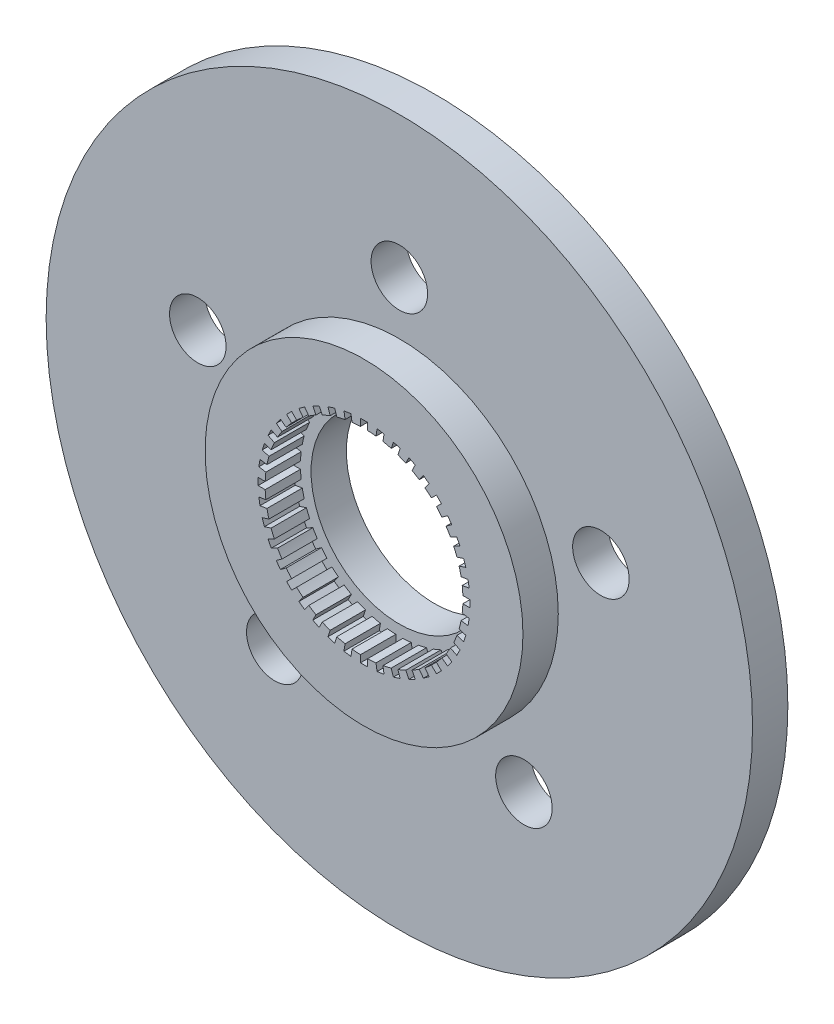
SolidWorks part; units mm, degrees
ref_plane "Front" through (0, 0, 0) normal (0, 0, 1) x (1, 0, 0)
ref_plane "Top" through (0, 0, 0) normal (0, 1, 0) x (1, 0, 0)
ref_plane "Right" through (0, 0, 0) normal (1, 0, 0) x (0, 0, -1)
sketch "草图1" plane through (0, 0, 0) normal (0, 0, 1) x (1, 0, 0)
  circle A0 centre (0, 0) radius 100
  circle A1 centre (0, 0) radius 25
  circle A2 centre (0, 60) radius 8
  circle A3 centre (57.0634, 18.541) radius 8
  circle A4 centre (35.2671, -48.541) radius 8
  circle A5 centre (-35.2671, -48.541) radius 8
  circle A6 centre (-57.0634, 18.541) radius 8
  point P17 (0, 0)
  dimension "D1" = 60
  dimension "D2" = 200
  dimension "D3" = 50
  dimension "D4" = 5
extrude "凸台-拉伸1" add sketch "草图1" along normal blind 10
sketch "草图2" plane through (0, 0, 10) normal (0, 0, 1) x (1, 0, 0)
  line L82 (3.3897, 27.7941) -> (3.7027, 29.7706)
  line L83 (-1, 27.9821) -> (-1, 29.9833)
  line L84 (-1, 29.9833) -> (1, 29.9833)
  line L85 (1, 29.9833) -> (1, 27.9821)
  line L86 (5.6781, 29.4577) -> (5.3651, 27.4812)
  line L87 (7.6959, 26.9216) -> (8.3143, 28.8249)
  line L88 (10.2164, 28.2068) -> (9.598, 26.3036)
  line L89 (11.8126, 25.3863) -> (12.7211, 27.1693)
  line L90 (14.5032, 26.2614) -> (13.5946, 24.4783)
  line L91 (15.6385, 23.2258) -> (16.8147, 24.8448)
  line L92 (18.4328, 23.6692) -> (17.2565, 22.0502)
  line L93 (19.0793, 20.4935) -> (20.4943, 21.9085)
  line L94 (21.9085, 20.4943) -> (20.4935, 19.0793)
  line L95 (22.0502, 17.2565) -> (23.6692, 18.4328)
  line L96 (24.8448, 16.8147) -> (23.2258, 15.6385)
  line L97 (24.4783, 13.5946) -> (26.2614, 14.5032)
  line L98 (27.1693, 12.7211) -> (25.3863, 11.8126)
  line L99 (26.3036, 9.598) -> (28.2068, 10.2164)
  line L100 (28.8249, 8.3143) -> (26.9216, 7.6959)
  line L101 (27.4812, 5.3651) -> (29.4577, 5.6781)
  line L102 (29.7706, 3.7027) -> (27.7941, 3.3897)
  line L103 (27.9821, 1) -> (29.9833, 1)
  line L104 (29.9833, -1) -> (27.9821, -1)
  line L105 (27.7941, -3.3897) -> (29.7706, -3.7027)
  line L106 (29.4577, -5.6781) -> (27.4812, -5.3651)
  line L107 (26.9216, -7.6959) -> (28.8249, -8.3143)
  line L108 (28.2068, -10.2164) -> (26.3036, -9.598)
  line L109 (25.3863, -11.8126) -> (27.1693, -12.7211)
  line L110 (26.2614, -14.5032) -> (24.4783, -13.5946)
  line L111 (23.2258, -15.6385) -> (24.8448, -16.8147)
  line L112 (23.6692, -18.4328) -> (22.0502, -17.2565)
  line L113 (20.4935, -19.0793) -> (21.9085, -20.4943)
  line L114 (20.4943, -21.9085) -> (19.0793, -20.4935)
  line L115 (17.2565, -22.0502) -> (18.4328, -23.6692)
  line L116 (16.8147, -24.8448) -> (15.6385, -23.2258)
  line L117 (13.5946, -24.4783) -> (14.5032, -26.2614)
  line L118 (12.7211, -27.1693) -> (11.8126, -25.3863)
  line L119 (9.598, -26.3036) -> (10.2164, -28.2068)
  line L120 (8.3143, -28.8249) -> (7.6959, -26.9216)
  line L121 (5.3651, -27.4812) -> (5.6781, -29.4577)
  line L122 (3.7027, -29.7706) -> (3.3897, -27.7941)
  line L123 (1, -27.9821) -> (1, -29.9833)
  line L124 (-1, -29.9833) -> (-1, -27.9821)
  line L125 (-3.3897, -27.7941) -> (-3.7027, -29.7706)
  line L126 (-5.6781, -29.4577) -> (-5.3651, -27.4812)
  line L127 (-7.6959, -26.9216) -> (-8.3143, -28.8249)
  line L128 (-10.2164, -28.2068) -> (-9.598, -26.3036)
  line L129 (-11.8126, -25.3863) -> (-12.7211, -27.1693)
  line L130 (-14.5032, -26.2614) -> (-13.5946, -24.4783)
  line L131 (-15.6385, -23.2258) -> (-16.8147, -24.8448)
  line L132 (-18.4328, -23.6692) -> (-17.2565, -22.0502)
  line L133 (-19.0793, -20.4935) -> (-20.4943, -21.9085)
  line L134 (-21.9085, -20.4943) -> (-20.4935, -19.0793)
  line L135 (-22.0502, -17.2565) -> (-23.6692, -18.4328)
  line L136 (-24.8448, -16.8147) -> (-23.2258, -15.6385)
  line L137 (-24.4783, -13.5946) -> (-26.2614, -14.5032)
  line L138 (-27.1693, -12.7211) -> (-25.3863, -11.8126)
  line L139 (-26.3036, -9.598) -> (-28.2068, -10.2164)
  line L140 (-28.8249, -8.3143) -> (-26.9216, -7.6959)
  line L141 (-27.4812, -5.3651) -> (-29.4577, -5.6781)
  line L142 (-29.7706, -3.7027) -> (-27.7941, -3.3897)
  line L143 (-27.9821, -1) -> (-29.9833, -1)
  line L144 (-29.9833, 1) -> (-27.9821, 1)
  line L145 (-27.7941, 3.3897) -> (-29.7706, 3.7027)
  line L146 (-29.4577, 5.6781) -> (-27.4812, 5.3651)
  line L147 (-26.9216, 7.6959) -> (-28.8249, 8.3143)
  line L148 (-28.2068, 10.2164) -> (-26.3036, 9.598)
  line L149 (-25.3863, 11.8126) -> (-27.1693, 12.7211)
  line L150 (-26.2614, 14.5032) -> (-24.4783, 13.5946)
  line L151 (-23.2258, 15.6385) -> (-24.8448, 16.8147)
  line L152 (-23.6692, 18.4328) -> (-22.0502, 17.2565)
  line L153 (-20.4935, 19.0793) -> (-21.9085, 20.4943)
  line L154 (-20.4943, 21.9085) -> (-19.0793, 20.4935)
  line L155 (-17.2565, 22.0502) -> (-18.4328, 23.6692)
  line L156 (-16.8147, 24.8448) -> (-15.6385, 23.2258)
  line L157 (-13.5946, 24.4783) -> (-14.5032, 26.2614)
  line L158 (-12.7211, 27.1693) -> (-11.8126, 25.3863)
  line L159 (-9.598, 26.3036) -> (-10.2164, 28.2068)
  line L160 (-8.3143, 28.8249) -> (-7.6959, 26.9216)
  line L161 (-5.3651, 27.4812) -> (-5.6781, 29.4577)
  line L162 (-3.7027, 29.7706) -> (-3.3897, 27.7941)
  line L163 (3.7027, 29.7706) -> (5.6781, 29.4577)
  line L164 (8.3143, 28.8249) -> (10.2164, 28.2068)
  line L165 (12.7211, 27.1693) -> (14.5032, 26.2614)
  line L166 (16.8147, 24.8448) -> (18.4328, 23.6692)
  line L167 (20.4943, 21.9085) -> (21.9085, 20.4943)
  line L168 (23.6692, 18.4328) -> (24.8448, 16.8147)
  line L169 (26.2614, 14.5032) -> (27.1693, 12.7211)
  line L170 (28.2068, 10.2164) -> (28.8249, 8.3143)
  line L171 (29.4577, 5.6781) -> (29.7706, 3.7027)
  line L172 (29.9833, 1) -> (29.9833, -1)
  line L173 (29.7706, -3.7027) -> (29.4577, -5.6781)
  line L174 (28.8249, -8.3143) -> (28.2068, -10.2164)
  line L175 (27.1693, -12.7211) -> (26.2614, -14.5032)
  line L176 (24.8448, -16.8147) -> (23.6692, -18.4328)
  line L177 (21.9085, -20.4943) -> (20.4943, -21.9085)
  line L178 (18.4328, -23.6692) -> (16.8147, -24.8448)
  line L179 (14.5032, -26.2614) -> (12.7211, -27.1693)
  line L180 (10.2164, -28.2068) -> (8.3143, -28.8249)
  line L181 (5.6781, -29.4577) -> (3.7027, -29.7706)
  line L182 (1, -29.9833) -> (-1, -29.9833)
  line L183 (-3.7027, -29.7706) -> (-5.6781, -29.4577)
  line L184 (-8.3143, -28.8249) -> (-10.2164, -28.2068)
  line L185 (-12.7211, -27.1693) -> (-14.5032, -26.2614)
  line L186 (-16.8147, -24.8448) -> (-18.4328, -23.6692)
  line L187 (-20.4943, -21.9085) -> (-21.9085, -20.4943)
  line L188 (-23.6692, -18.4328) -> (-24.8448, -16.8147)
  line L189 (-26.2614, -14.5032) -> (-27.1693, -12.7211)
  line L190 (-28.2068, -10.2164) -> (-28.8249, -8.3143)
  line L191 (-29.4577, -5.6781) -> (-29.7706, -3.7027)
  line L192 (-29.9833, -1) -> (-29.9833, 1)
  line L193 (-29.7706, 3.7027) -> (-29.4577, 5.6781)
  line L194 (-28.8249, 8.3143) -> (-28.2068, 10.2164)
  line L195 (-27.1693, 12.7211) -> (-26.2614, 14.5032)
  line L196 (-24.8448, 16.8147) -> (-23.6692, 18.4328)
  line L197 (-21.9085, 20.4943) -> (-20.4943, 21.9085)
  line L198 (-18.4328, 23.6692) -> (-16.8147, 24.8448)
  line L199 (-14.5032, 26.2614) -> (-12.7211, 27.1693)
  line L200 (-10.2164, 28.2068) -> (-8.3143, 28.8249)
  line L201 (-5.6781, 29.4577) -> (-3.7027, 29.7706)
  arc A84 (-1, 27.9821) -> (-3.3897, 27.7941) centre (0, 0) ccw
  circle A85 centre (0, 0) radius 45
  arc A87 (3.3897, 27.7941) -> (1, 27.9821) centre (0, 0) ccw
  arc A88 (7.6959, 26.9216) -> (5.3651, 27.4812) centre (0, 0) ccw
  arc A89 (11.8126, 25.3863) -> (9.598, 26.3036) centre (0, 0) ccw
  arc A90 (15.6385, 23.2258) -> (13.5946, 24.4783) centre (0, 0) ccw
  arc A91 (19.0793, 20.4935) -> (17.2565, 22.0502) centre (0, 0) ccw
  arc A92 (22.0502, 17.2565) -> (20.4935, 19.0793) centre (0, 0) ccw
  arc A93 (24.4783, 13.5946) -> (23.2258, 15.6385) centre (0, 0) ccw
  arc A94 (26.3036, 9.598) -> (25.3863, 11.8126) centre (0, 0) ccw
  arc A95 (27.4812, 5.3651) -> (26.9216, 7.6959) centre (0, 0) ccw
  arc A96 (27.9821, 1) -> (27.7941, 3.3897) centre (0, 0) ccw
  arc A97 (27.7941, -3.3897) -> (27.9821, -1) centre (0, 0) ccw
  arc A98 (26.9216, -7.6959) -> (27.4812, -5.3651) centre (0, 0) ccw
  arc A99 (25.3863, -11.8126) -> (26.3036, -9.598) centre (0, 0) ccw
  arc A100 (23.2258, -15.6385) -> (24.4783, -13.5946) centre (0, 0) ccw
  arc A101 (20.4935, -19.0793) -> (22.0502, -17.2565) centre (0, 0) ccw
  arc A102 (17.2565, -22.0502) -> (19.0793, -20.4935) centre (0, 0) ccw
  arc A103 (13.5946, -24.4783) -> (15.6385, -23.2258) centre (0, 0) ccw
  arc A104 (9.598, -26.3036) -> (11.8126, -25.3863) centre (0, 0) ccw
  arc A105 (5.3651, -27.4812) -> (7.6959, -26.9216) centre (0, 0) ccw
  arc A106 (1, -27.9821) -> (3.3897, -27.7941) centre (0, 0) ccw
  arc A107 (-3.3897, -27.7941) -> (-1, -27.9821) centre (0, 0) ccw
  arc A108 (-7.6959, -26.9216) -> (-5.3651, -27.4812) centre (0, 0) ccw
  arc A109 (-11.8126, -25.3863) -> (-9.598, -26.3036) centre (0, 0) ccw
  arc A110 (-15.6385, -23.2258) -> (-13.5946, -24.4783) centre (0, 0) ccw
  arc A111 (-19.0793, -20.4935) -> (-17.2565, -22.0502) centre (0, 0) ccw
  arc A112 (-22.0502, -17.2565) -> (-20.4935, -19.0793) centre (0, 0) ccw
  arc A113 (-24.4783, -13.5946) -> (-23.2258, -15.6385) centre (0, 0) ccw
  arc A114 (-26.3036, -9.598) -> (-25.3863, -11.8126) centre (0, 0) ccw
  arc A115 (-27.4812, -5.3651) -> (-26.9216, -7.6959) centre (0, 0) ccw
  arc A116 (-27.9821, -1) -> (-27.7941, -3.3897) centre (0, 0) ccw
  arc A117 (-27.7941, 3.3897) -> (-27.9821, 1) centre (0, 0) ccw
  arc A118 (-26.9216, 7.6959) -> (-27.4812, 5.3651) centre (0, 0) ccw
  arc A119 (-25.3863, 11.8126) -> (-26.3036, 9.598) centre (0, 0) ccw
  arc A120 (-23.2258, 15.6385) -> (-24.4783, 13.5946) centre (0, 0) ccw
  arc A121 (-20.4935, 19.0793) -> (-22.0502, 17.2565) centre (0, 0) ccw
  arc A122 (-17.2565, 22.0502) -> (-19.0793, 20.4935) centre (0, 0) ccw
  arc A123 (-13.5946, 24.4783) -> (-15.6385, 23.2258) centre (0, 0) ccw
  arc A124 (-9.598, 26.3036) -> (-11.8126, 25.3863) centre (0, 0) ccw
  arc A125 (-5.3651, 27.4812) -> (-7.6959, 26.9216) centre (0, 0) ccw
extrude "凸台-拉伸2" add sketch "草图2" along normal blind 20 from surface at -10 starting at face at (100, 0, 0)
